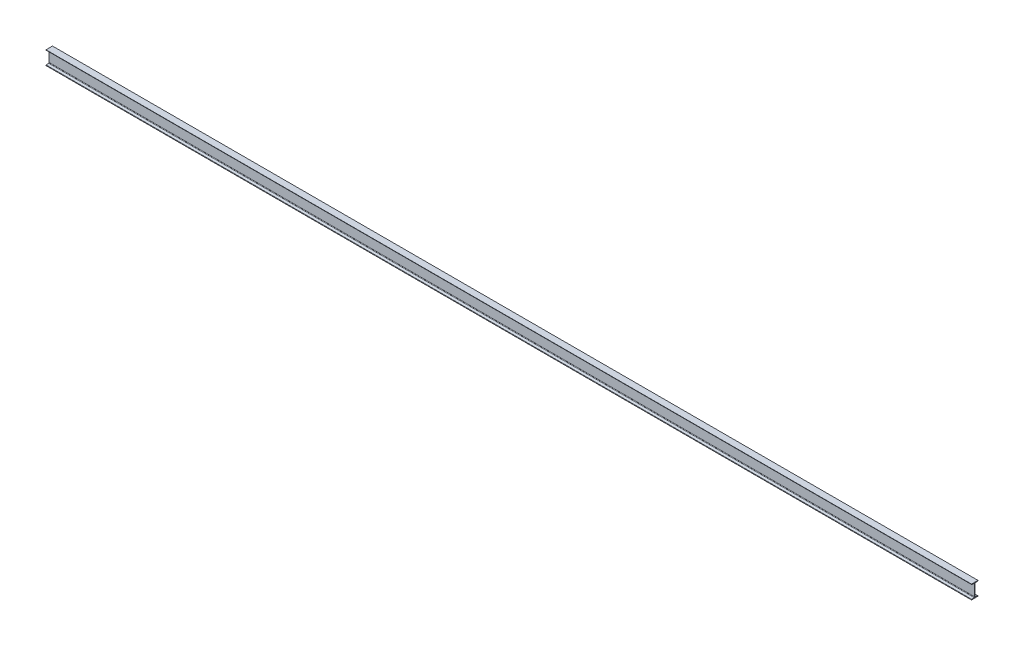
from build123d import *

# Parameters (mm, degrees)
BASE_DEPTH = 16840
FILLET1_R  = 10
FILLET2_R  = 5


with BuildPart() as part:
    # Sketch1 → Base (new body)
    with BuildSketch(Plane(origin=(0, 0, 0), x_dir=(0, 0, -1), z_dir=(1, 0, 0))):
        Polygon((-59, 0), (59, 0), (59, 7.666666667), (5, 16.666666667), (5, 233.333333333), (59, 242.333333333), (59, 250), (-59, 250), (-59, 242.333333333), (-5, 233.333333333), (-5, 16.666666667), (-59, 7.666666667), align=None)
    extrude(amount=BASE_DEPTH)

    # Fillet1
    fillet1_edges = [part.edges().sort_by_distance(p)[0] for p in [
        (8420, 16.666666667, 5),
        (8420, 233.333333333, 5),
        (8420, 233.333333333, -5),
        (8420, 16.666666667, -5),
    ]]
    fillet(fillet1_edges, radius=FILLET1_R)

    # Fillet2
    fillet2_edges = [part.edges().sort_by_distance(p)[0] for p in [
        (8420, 7.666666667, 59),
        (8420, 242.333333333, 59),
        (8420, 242.333333333, -59),
        (8420, 7.666666667, -59),
    ]]
    fillet(fillet2_edges, radius=FILLET2_R)


solid = part.part
